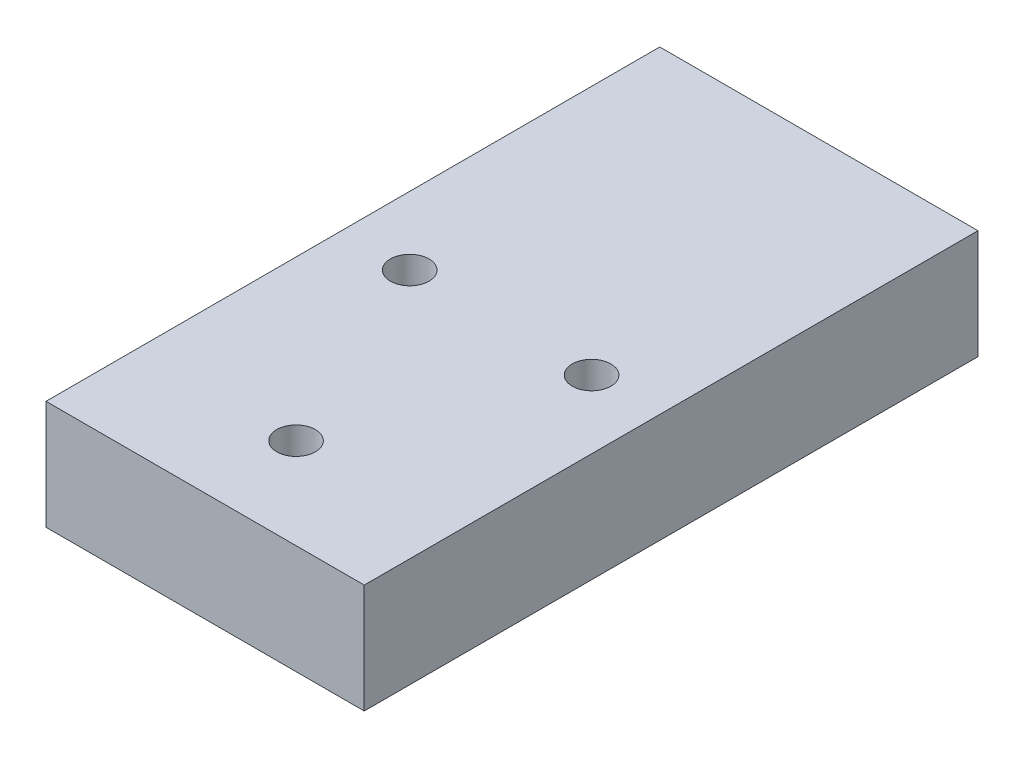
SolidWorks part; units mm, degrees
material "A3"
ref_plane "前视基准面" through (0, 0, 0) normal (0, 0, 1) x (1, 0, 0)
ref_plane "上视基准面" through (0, 0, 0) normal (0, 1, 0) x (1, 0, 0)
ref_plane "右视基准面" through (0, 0, 0) normal (1, 0, 0) x (0, 0, -1)
sketch "草图1" plane through (0, 0, 0) normal (0, 1, 0) x (1, 0, 0)
  line L1 (-35, -67.5) -> (35, -67.5)
  line L2 (-35, -67.5) -> (-35, 67.5)
  line L3 (-35, 67.5) -> (35, 67.5)
  line L4 (35, -67.5) -> (35, 67.5)
  line L5 (-35, -67.5) -> (35, 67.5) construction
  line L6 (-35, 67.5) -> (35, -67.5) construction
  point P0 (0, 0)
  dimension "D1" = 135
  dimension "D2" = 70
extrude "凸台-拉伸1" add sketch "草图1" along normal blind 24
hole_wizard "M10 螺纹孔1" positions "草图2" profile "草图3" tap size "M10" standard "GB" end condition through all
sketch "草图2" plane through (0, 24, 0) normal (0, 1, 0) x (1, 0, 0)
  line L0 (0, 67.5) -> (0, -2.5) construction
  line L1 (35, 67.5) -> (-35, 67.5) construction
  line L2 (0, -2.5) -> (45, -2.5) construction
  line L4 (-35, -67.5) -> (35, -67.5) construction
  point P0 (-20, -2.5)
  point P16 (20, -2.5)
  point P18 (0, -47.5)
  dimension "D1" = 40
  dimension "D2" = 20
  dimension "D3" = 45
sketch "草图3" plane through (-20, 24, 2.5) normal (1, 0, 0) x (0, 0, 1)
  line L0 (0, 0) -> (0, 24)
  line L1 (0, 24) -> (4.25, 24)
  line L2 (4.25, 24) -> (4.25, 0)
  line L5 (4.25, 0) -> (0, 0)
  line L11 (0, -6.35) -> (0, 107.95) construction
  dimension "通孔螺纹孔钻头直径" = 8.5
  dimension "通孔螺纹孔钻头深度" = 24
cosmetic thread "孔螺蚊线1"
cosmetic thread "孔螺蚊线2"
cosmetic thread "孔螺蚊线4"
